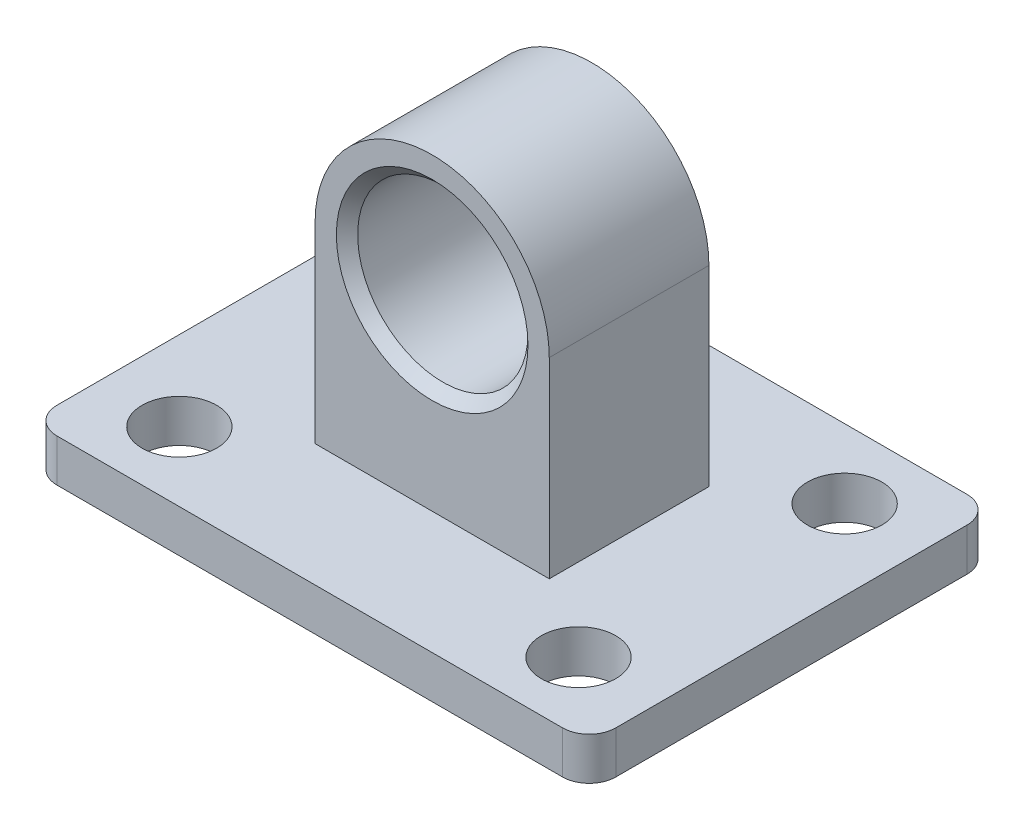
SolidWorks part; units mm, degrees
material "A3"
ref_plane "前视基准面" through (0, 0, 0) normal (0, 0, 1) x (1, 0, 0)
ref_plane "上视基准面" through (0, 0, 0) normal (0, 1, 0) x (1, 0, 0)
ref_plane "右视基准面" through (0, 0, 0) normal (1, 0, 0) x (0, 0, -1)
sketch "草图1" plane through (0, 0, 0) normal (0, 1, 0) x (1, 0, 0)
  line L0 (0, 38) -> (0, 0) construction
  line L1 (-47.5, -38) -> (47.5, -38)
  line L2 (-52.5, -33) -> (-52.5, 33)
  line L3 (-47.5, 38) -> (47.5, 38)
  line L4 (52.5, -33) -> (52.5, 33)
  line L5 (-52.5, -38) -> (52.5, 38) construction
  line L6 (-52.5, 38) -> (52.5, -38) construction
  line L7 (0, 0) -> (52.5, 0) construction
  arc A0 (47.5, -38) -> (52.5, -33) centre (47.5, -33) ccw
  arc A1 (-52.5, 33) -> (-47.5, 38) centre (-47.5, 33) cw
  arc A2 (-47.5, -38) -> (-52.5, -33) centre (-47.5, -33) cw
  arc A3 (47.5, 38) -> (52.5, 33) centre (47.5, 33) cw
  circle A4 centre (-37.5, -25) radius 7
  circle A5 centre (37.5, -25) radius 7
  circle A6 centre (-37.5, 25) radius 7
  circle A7 centre (37.5, 25) radius 7
  point P0 (0, 0)
  dimension "D3" = 5
  dimension "D4" = 14
  dimension "D5" = 37.5
  dimension "D6" = 25
  dimension "D1" = 76
  dimension "D2" = 105
extrude "凸台-拉伸1" add sketch "草图1" along normal blind 8
sketch "草图2" plane through (0, 0, 0) normal (0, 0, 1) x (1, 0, 0)
  line L0 (-47.5, 8) -> (47.5, 8) construction
  line L1 (-22, 44) -> (22, 44) construction
  line L2 (-22, 44) -> (-22, 8)
  line L3 (-22, 8) -> (22, 8)
  line L4 (22, 44) -> (22, 8)
  line L5 (-22, 44) -> (22, 8) construction
  line L6 (-22, 8) -> (22, 44) construction
  line L7 (-47.5, 0) -> (47.5, 0) construction
  arc A1 (22, 44) -> (-22, 44) centre (0, 44) ccw
  circle A2 centre (0, 44) radius 16
  point P0 (0, 26)
  dimension "D3" = 32
  dimension "D1" = 44
  dimension "D2" = 44
extrude "凸台-拉伸2" add sketch "草图2" against normal mid plane 30 separate body
chamfer "倒角1" distance 2 angle 45 2 edges at (16, 44, 15) (16, 44, -15)
